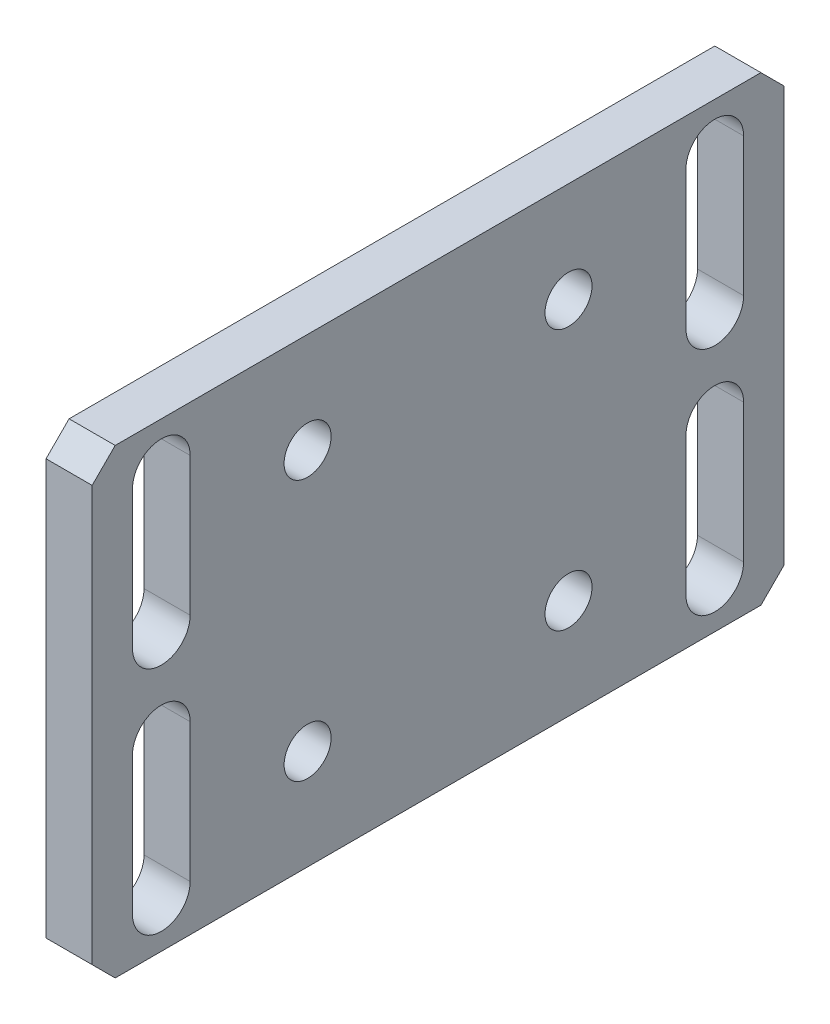
SolidWorks part; units mm, degrees
ref_plane "前视基准面" through (0, 0, 0) normal (0, 0, 1) x (1, 0, 0)
ref_plane "上视基准面" through (0, 0, 0) normal (0, 1, 0) x (1, 0, 0)
ref_plane "右视基准面" through (0, 0, 0) normal (1, 0, 0) x (0, 0, -1)
sketch "草图1" plane through (0, 0, 0) normal (1, 0, 0) x (0, 0, -1)
  line L1 (-75, 50) -> (75, 50)
  line L2 (-75, 50) -> (-75, -50)
  line L3 (-75, -50) -> (75, -50)
  line L4 (75, 50) -> (75, -50)
  line L5 (-75, 50) -> (75, -50) construction
  line L6 (-75, -50) -> (75, 50) construction
  point P0 (0, 0)
  dimension "D1" = 150
  dimension "D2" = 100
extrude "凸台-拉伸1" add sketch "草图1" along normal blind 10
hole_wizard "M12 螺纹孔1" positions "草图2" profile "草图3" tap size "M12" standard "GB" end condition through all
sketch "草图2" plane through (10, 0, 0) normal (1, 0, 0) x (0, 0, -1)
  line L0 (0, 0) -> (-28.2843, 28.2843) construction
  line L2 (0, 0) -> (0, 22.1893) construction
  point P0 (-28.2843, 28.2843)
  point P18 (28.2843, 28.2843)
  point P19 (28.2843, -28.2843)
  point P20 (-28.2843, -28.2843)
  dimension "D1" = 45
  dimension "D2" = 40
  dimension "D3" = 4
sketch "草图3" plane through (10, 28.2843, 28.2843) normal (0, 1, 0) x (0, 0, -1)
  line L0 (0, 0) -> (0, 10)
  line L1 (0, 10) -> (5.1, 10)
  line L2 (5.1, 10) -> (5.1, 0)
  line L5 (5.1, 0) -> (0, 0)
  line L11 (0, -6.35) -> (0, 107.95) construction
  dimension "通孔螺纹孔钻头直径" = 10.2
  dimension "通孔螺纹孔钻头深度" = 10
cosmetic thread "孔螺蚊线1" parameters "D2"=12
cosmetic thread "孔螺蚊线2" parameters "D2"=12
cosmetic thread "孔螺蚊线3" parameters "D2"=12
cosmetic thread "孔螺蚊线4" parameters "D2"=12
sketch "草图4" plane through (10, 0, 0) normal (1, 0, 0) x (0, 0, -1)
  line L0 (-60, 40) -> (-60, 10) construction
  line L1 (-53.75, 40) -> (-53.75, 10)
  line L2 (-66.25, 40) -> (-66.25, 10)
  line L3 (0, 77.9434) -> (0, 0) construction
  line L4 (0, 0) -> (127.0456, 0) construction
  line L5 (60, 40) -> (60, 10) construction
  line L6 (53.75, 40) -> (53.75, 10)
  line L7 (66.25, 40) -> (66.25, 10)
  line L8 (-60, -40) -> (-60, -10) construction
  line L9 (-53.75, -40) -> (-53.75, -10)
  line L10 (-66.25, -40) -> (-66.25, -10)
  line L11 (60, -40) -> (60, -10) construction
  line L12 (53.75, -40) -> (53.75, -10)
  line L13 (66.25, -40) -> (66.25, -10)
  arc A0 (-53.75, 40) -> (-66.25, 40) centre (-60, 40) ccw
  arc A1 (-66.25, 10) -> (-53.75, 10) centre (-60, 10) ccw
  arc A2 (53.75, 40) -> (66.25, 40) centre (60, 40) cw
  arc A3 (66.25, 10) -> (53.75, 10) centre (60, 10) cw
  arc A4 (-53.75, -40) -> (-66.25, -40) centre (-60, -40) cw
  arc A5 (-66.25, -10) -> (-53.75, -10) centre (-60, -10) cw
  arc A6 (53.75, -40) -> (66.25, -40) centre (60, -40) ccw
  arc A7 (66.25, -10) -> (53.75, -10) centre (60, -10) ccw
  point P2 (-60, 25)
  point P13 (60, 25)
  point P20 (-60, -25)
  point P27 (60, -25)
  dimension "D1" = 30
  dimension "D2" = 120
  dimension "D3" = 50
  dimension "D4" = 12.5
extrude "切除-拉伸1" cut sketch "草图4" against normal through all
chamfer "倒角1" distance 5 angle 45 4 edges at (5, -50, 75) (5, 50, 75) (5, 50, -75) (5, -50, -75)
